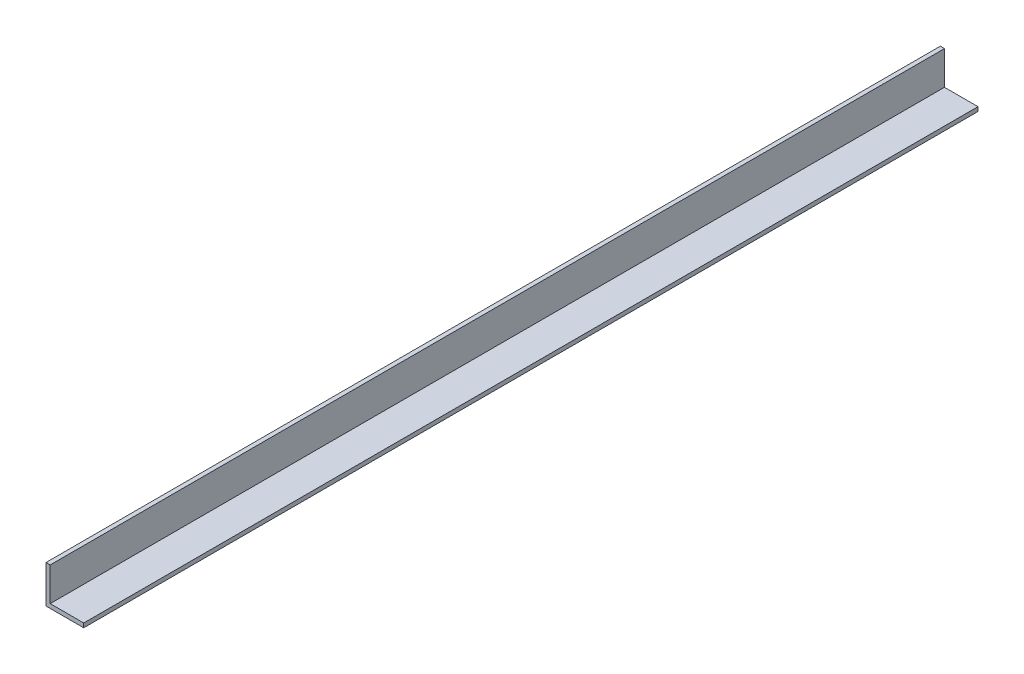
from build123d import *

# Parameters (mm, degrees)
EXTRUDE1_DEPTH = 1066.8


with BuildPart() as part:
    # Sketch1 → Extrude1 (new body)
    with BuildSketch(Plane.XY):
        Polygon((-24.649517418, 21.952701214), (-24.649517418, -23.047298786), (20.350482582, -23.047298786), (20.350482582, -18.047298786), (-19.649517418, -18.047298786), (-19.649517418, 21.952701214), align=None)
    extrude(amount=EXTRUDE1_DEPTH)


solid = part.part
